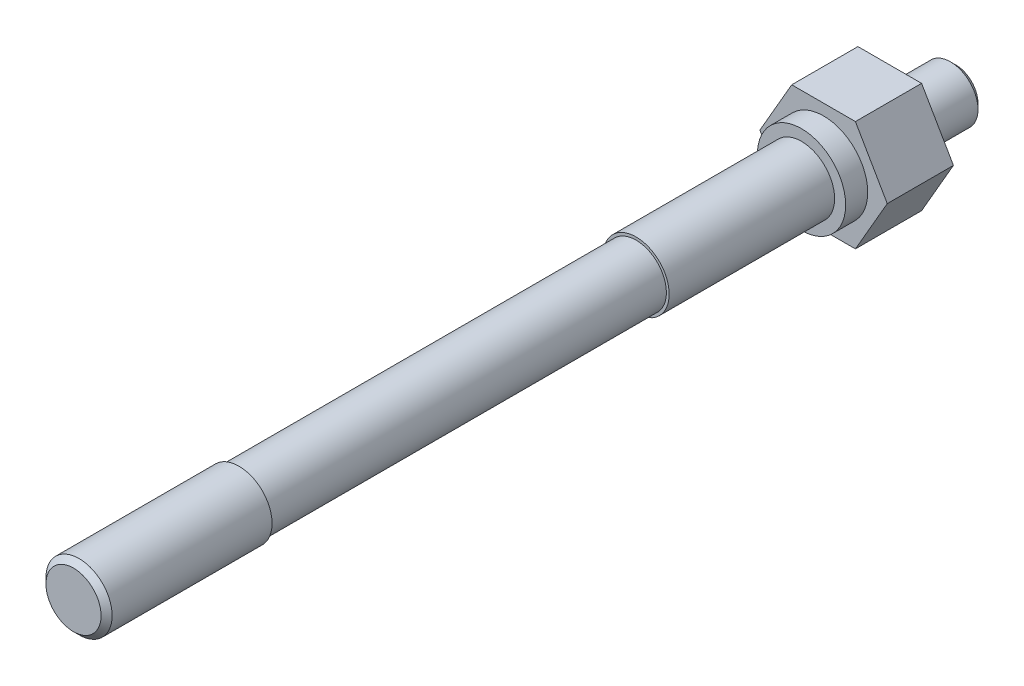
SolidWorks part; units mm, degrees
ref_plane "Front Plane" through (0, 0, 0) normal (0, 0, 1) x (1, 0, 0)
ref_plane "Top Plane" through (0, 0, 0) normal (0, 1, 0) x (1, 0, 0)
ref_plane "Right Plane" through (0, 0, 0) normal (1, 0, 0) x (0, 0, -1)
sketch "Sketch1" plane through (0, 0, 0) normal (0, 0, 1) x (1, 0, 0)
  line L1 (5.7735, 0) -> (2.8868, 5)
  line L2 (2.8868, 5) -> (-2.8868, 5)
  line L3 (-2.8868, 5) -> (-5.7735, 0)
  line L4 (-5.7735, 0) -> (-2.8868, -5)
  line L5 (-2.8868, -5) -> (2.8868, -5)
  line L6 (2.8868, -5) -> (5.7735, 0)
  circle A0 centre (0, 0) radius 5 construction
  dimension "D1" = 10
extrude "Boss-Extrude1" add sketch "Sketch1" along normal blind 6
sketch "Sketch2" plane through (0, 0, 0) normal (0, 0, -1) x (-1, 0, 0)
  circle A0 centre (0, 0) radius 2.5
  dimension "D1" = 5
extrude "Boss-Extrude2" add sketch "Sketch2" along normal blind 6
cosmetic thread "Cosmetic Thread1" parameters "D2"=4.134
sketch "Sketch3" plane through (0, 0, 6) normal (0, 0, 1) x (1, 0, 0)
  circle A0 centre (0, 0) radius 4
  dimension "D1" = 8
extrude "Boss-Extrude3" add sketch "Sketch3" along normal blind 2
sketch "Sketch4" plane through (0, 0, 8) normal (0, 0, 1) x (1, 0, 0)
  circle A0 centre (0, 0) radius 3
  dimension "D1" = 6
extrude "Boss-Extrude4" add sketch "Sketch4" along normal blind 66
chamfer "Chamfer1" distance 0.5 angle 45 1 edges at (3, 0, 74)
ref_axis "Axis1" through (0, 0, 73.5) along (0, 0, -1)
sketch "Sketch5" plane through (0, 0, 0) normal (0, 1, 0) x (1, 0, 0)
  line L0 (-3, -8) -> (3, -8) construction
  line L1 (2.75, -23) -> (7.75, -23)
  line L2 (2.75, -23) -> (2.75, -59)
  line L3 (2.75, -59) -> (7.75, -59)
  line L4 (7.75, -23) -> (7.75, -59)
  line L5 (-2.5, -74) -> (2.5, -74) construction
  line L6 (3, -73.5) -> (3, -8) construction
  dimension "D1" = 15
  dimension "D2" = 15
  dimension "D3" = 0.25
  dimension "D4" = 5
revolve "Cut-Revolve1" cut sketch "Sketch5" angle 360 about axis through (0, 0, 73.5) along (0, 0, -1)
chamfer "Chamfer2" distance 0.5 angle 45 1 edges at (-2.5, 0, -6)
